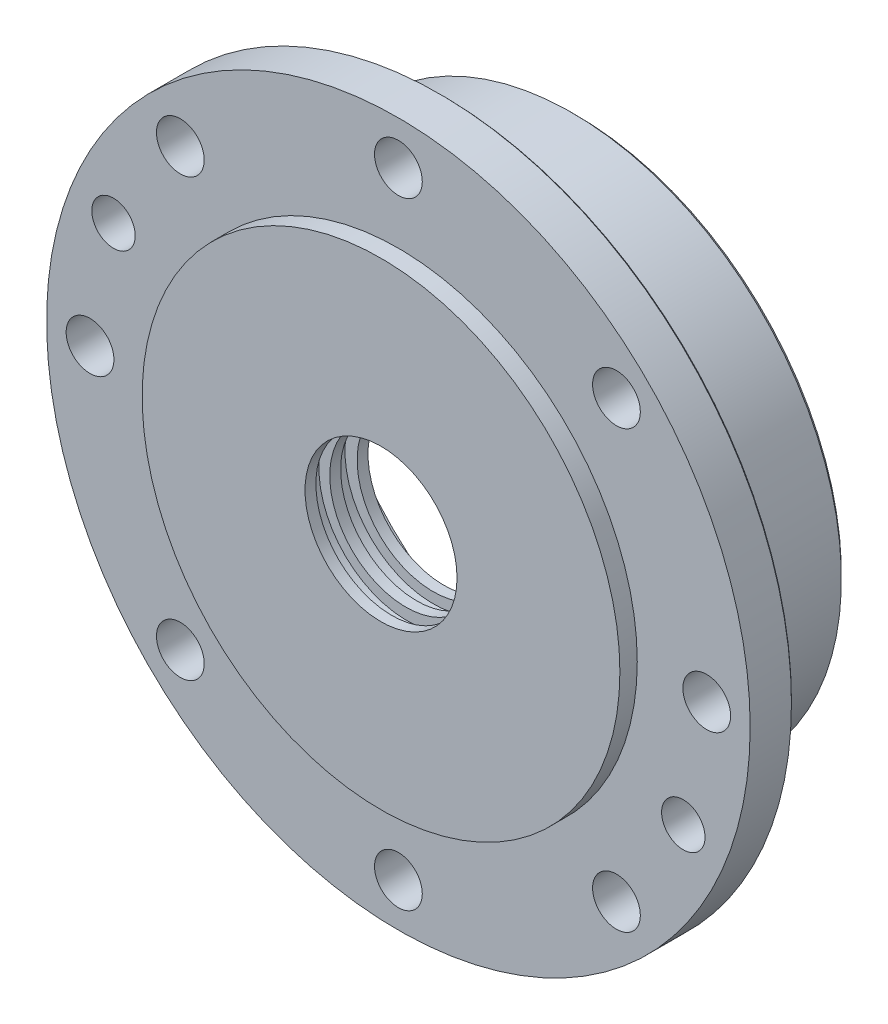
from build123d import *

# Parameters (mm, degrees)
SKETCH1_R                    = 81
BOSS_EXTRUDE1_DEPTH          = 10
SKETCH2_R                    = 55
BOSS_EXTRUDE2_DEPTH          = 4
SKETCH3_R                    = 62
BOSS_EXTRUDE3_DEPTH          = 31
SKETCH4_R                    = 17.5
CUT_EXTRUDE1_DEPTH           = 2.5
SKETCH5_R                    = 20.3
CUT_EXTRUDE2_DEPTH           = 3.5
SKETCH6_R                    = 17.5
CUT_EXTRUDE3_DEPTH           = 2.5
SKETCH7_R                    = 20.3
CUT_EXTRUDE4_DEPTH           = 3.5
SKETCH8_R                    = 17.5
CUT_EXTRUDE5_DEPTH           = 2.5
SKETCH9_R                    = 50
CUT_EXTRUDE6_DEPTH           = 1.5
F_1_0MM_BLIND_DOWEL_HOLE1_D  = 11
CIRPATTERN1_COUNT            = 8
F_10_0MM_BLIND_DOWEL_HOLE1_D = 10
SKETCH18_R                   = 58
CUT_EXTRUDE7_DEPTH           = 4
SKETCH19_R                   = 60
CUT_EXTRUDE8_DEPTH           = 9
SKETCH20_R                   = 60.5
CUT_EXTRUDE9_DEPTH           = 3
CUT_EXTRUDE10_REACH          = 121.21
SKETCH21_R                   = 57.5
CHAMFER1_SIZE                = 1
CHAMFER2_SIZE                = 0.5


with BuildPart() as part:
    # Sketch1 → Boss-Extrude1 (new body)
    with BuildSketch(Plane.XY):
        Circle(SKETCH1_R)
    extrude(amount=BOSS_EXTRUDE1_DEPTH)

    # Sketch2 → Boss-Extrude2 (add)
    with BuildSketch(Plane.XY.offset(10)):
        Circle(SKETCH2_R)
    extrude(amount=BOSS_EXTRUDE2_DEPTH)

    # Sketch3 → Boss-Extrude3 (add)
    with BuildSketch(Plane(origin=(0, 0, 0), x_dir=(-1, 0, 0), z_dir=(0, 0, -1))):
        Circle(SKETCH3_R)
    extrude(amount=BOSS_EXTRUDE3_DEPTH)

    # Sketch4 → Cut-Extrude1 (cut)
    with BuildSketch(Plane.XY.offset(14)):
        Circle(SKETCH4_R)
    extrude(amount=-CUT_EXTRUDE1_DEPTH, mode=Mode.SUBTRACT)

    # Sketch5 → Cut-Extrude2 (cut)
    with BuildSketch(Plane.XY.offset(11.5)):
        Circle(SKETCH5_R)
    extrude(amount=-CUT_EXTRUDE2_DEPTH, mode=Mode.SUBTRACT)

    # Sketch6 → Cut-Extrude3 (cut)
    with BuildSketch(Plane.XY.offset(8)):
        with Locations((-0.303631116, -0.227723337)):
            Circle(SKETCH6_R)
    extrude(amount=-CUT_EXTRUDE3_DEPTH, mode=Mode.SUBTRACT)

    # Sketch7 → Cut-Extrude4 (cut)
    with BuildSketch(Plane.XY.offset(5.5)):
        with Locations((0, 0.379538895)):
            Circle(SKETCH7_R)
    extrude(amount=-CUT_EXTRUDE4_DEPTH, mode=Mode.SUBTRACT)

    # Sketch8 → Cut-Extrude5 (cut)
    with BuildSketch(Plane.XY.offset(2)):
        Circle(SKETCH8_R)
    extrude(amount=-CUT_EXTRUDE5_DEPTH, mode=Mode.SUBTRACT)

    # Sketch9 → Cut-Extrude6 (cut)
    with BuildSketch(Plane.XY.offset(-0.5)):
        Circle(SKETCH9_R)
    extrude(amount=-CUT_EXTRUDE6_DEPTH, mode=Mode.SUBTRACT)

    # Ø1.0mm Blind Dowel Hole1 (through all)
    with Locations(Plane.XY.offset(10)):
        with Locations((0, 71)):
            f_1_0mm_blind_dowel_hole1 = Hole(F_1_0MM_BLIND_DOWEL_HOLE1_D / 2)

    # CirPattern1: Ø1.0mm Blind Dowel Hole1 ×8 about axis
    cirpattern1_axis = Axis((0, 0, 0), (0, 0, 1))
    for i in range(1, CIRPATTERN1_COUNT):
        add(f_1_0mm_blind_dowel_hole1.rotate(cirpattern1_axis, i * 360 / CIRPATTERN1_COUNT), mode=Mode.SUBTRACT)

    # Ø10.0mm Blind Dowel Hole1 (through all)
    with Locations(Plane.XY.offset(10)):
        with Locations((65.595446808, -27.170523698), (-65.595446808, 27.170523698)):
            Hole(F_10_0MM_BLIND_DOWEL_HOLE1_D / 2)

    # Sketch18 → Cut-Extrude7 (cut)
    with BuildSketch(Plane.XY.offset(-2)):
        Circle(SKETCH18_R)
    extrude(amount=-CUT_EXTRUDE7_DEPTH, mode=Mode.SUBTRACT)

    # Sketch19 → Cut-Extrude8 (cut)
    with BuildSketch(Plane(origin=(0, 0, -31), x_dir=(-1, 0, 0), z_dir=(0, 0, -1))):
        Circle(SKETCH19_R)
    extrude(amount=-CUT_EXTRUDE8_DEPTH, mode=Mode.SUBTRACT)

    # Sketch20 → Cut-Extrude9 (cut)
    with BuildSketch(Plane(origin=(0, 0, -22), x_dir=(-1, 0, 0), z_dir=(0, 0, -1))):
        Circle(SKETCH20_R)
    extrude(amount=-CUT_EXTRUDE9_DEPTH, mode=Mode.SUBTRACT)

    # Sketch21 → Cut-Extrude10 (cut, up to next)
    with BuildSketch(Plane(origin=(0, 0, -19), x_dir=(-1, 0, 0), z_dir=(0, 0, -1)), mode=Mode.PRIVATE) as cut_extrude10_sk1:
        Circle(SKETCH21_R)
    cut_extrude10_tool1 = extrude(cut_extrude10_sk1.sketch, amount=-CUT_EXTRUDE10_REACH, mode=Mode.PRIVATE) & part.part
    add(cut_extrude10_tool1.solids().sort_by_distance((0, 0, -19))[0], mode=Mode.SUBTRACT)

    # Chamfer1
    chamfer1_edges = [part.edges().sort_by_distance(p)[0] for p in [
        (62, 0, -31),
    ]]
    chamfer(chamfer1_edges, length=CHAMFER1_SIZE)

    # Chamfer2
    chamfer2_edges = [part.edges().sort_by_distance(p)[0] for p in [
        (-81, 0, 0),
    ]]
    chamfer(chamfer2_edges, length=CHAMFER2_SIZE)


solid = part.part
